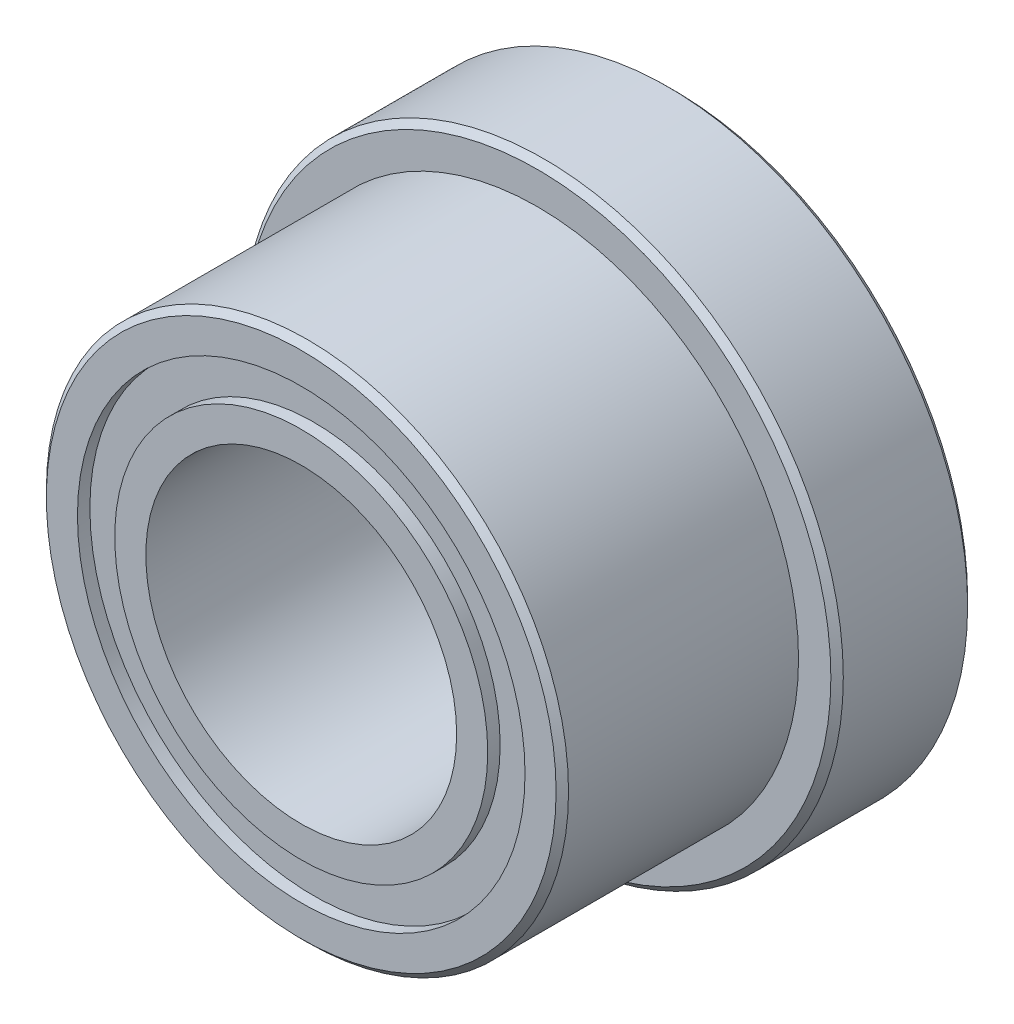
from build123d import *

# Parameters (mm, degrees)
SKETCH1_R           = 24.1
BOSS_EXTRUDE1_DEPTH = 11
SKETCH2_R           = 15
CUT_EXTRUDE1_DEPTH  = 36.813684535
SKETCH3_R           = 21
SKETCH3_R_2         = 12.5
BOSS_EXTRUDE2_DEPTH = 19
CHAMFER1_SIZE       = 0.5
SKETCH4_R           = 18
SKETCH4_R_2         = 15
CUT_EXTRUDE2_DEPTH  = 1


with BuildPart() as part:
    # Sketch1 → Boss-Extrude1 (new body)
    with BuildSketch(Plane.XY):
        Circle(SKETCH1_R)
    extrude(amount=BOSS_EXTRUDE1_DEPTH)

    # Sketch2 → Cut-Extrude1 (cut, through all)
    with BuildSketch(Plane.XY.offset(11)):
        Circle(SKETCH2_R)
    extrude(amount=-CUT_EXTRUDE1_DEPTH, mode=Mode.SUBTRACT)

    # Sketch3 → Boss-Extrude2 (add)
    with BuildSketch(Plane.XY.offset(11)):
        Circle(SKETCH3_R)
        Circle(SKETCH3_R_2, mode=Mode.SUBTRACT)
    extrude(amount=BOSS_EXTRUDE2_DEPTH)

    # Chamfer1
    chamfer1_edges = [part.edges().sort_by_distance(p)[0] for p in [
        (-21, 0, 30),
        (-24.1, 0, 0),
        (-24.1, 0, 11),
    ]]
    chamfer(chamfer1_edges, length=CHAMFER1_SIZE)

    # Sketch4 → Cut-Extrude2 (cut)
    with BuildSketch(Plane.XY.offset(30)):
        Circle(SKETCH4_R)
        Circle(SKETCH4_R_2, mode=Mode.SUBTRACT)
    extrude(amount=-CUT_EXTRUDE2_DEPTH, mode=Mode.SUBTRACT)


solid = part.part
